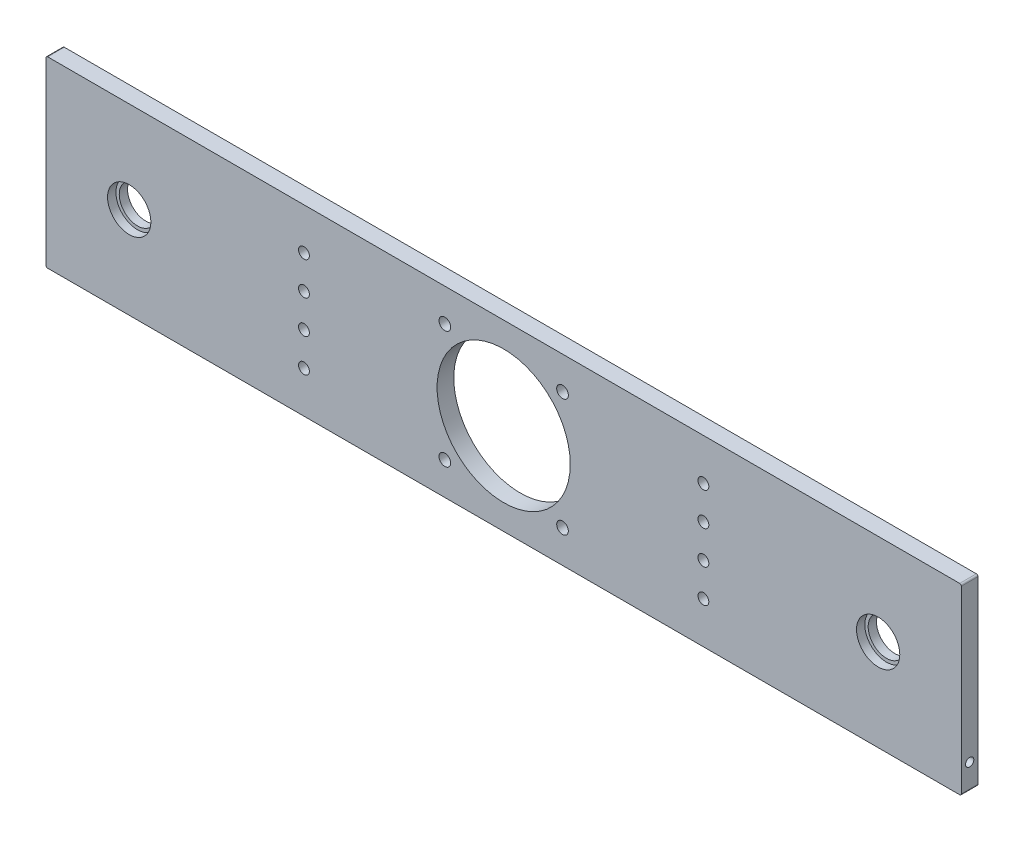
from build123d import *

# Parameters (mm, degrees)
SKETCH1_W           = 550
SKETCH1_H           = 110
BOSS_EXTRUDE1_DEPTH = 10
SKETCH3_R           = 13
CUT_EXTRUDE2_DEPTH  = 5
SKETCH4_R           = 11
CUT_EXTRUDE3_DEPTH  = 281.490641555
SKETCH5_R           = 40
CUT_EXTRUDE4_DEPTH  = 281.624304008
SKETCH6_R           = 3.5
CUT_EXTRUDE5_DEPTH  = 281.624304008
SKETCH7_R           = 3.25
CUT_EXTRUDE6_DEPTH  = 281.624304008
FILLET1_R           = 1


with BuildPart() as part:
    # Sketch1 → Boss-Extrude1 (new body)
    with BuildSketch(Plane.XY):
        Rectangle(SKETCH1_W, SKETCH1_H)
    extrude(amount=BOSS_EXTRUDE1_DEPTH)

    # Sketch3 → Cut-Extrude2 (cut)
    with BuildSketch(Plane.XY.offset(10)):
        with Locations((225, 0)):
            Circle(SKETCH3_R)
        with Locations(Location((-225, 0, 0), (0, 0, 180))):
            Circle(SKETCH3_R)
    extrude(amount=-CUT_EXTRUDE2_DEPTH, mode=Mode.SUBTRACT)

    # Sketch4 → Cut-Extrude3 (cut, through all)
    with BuildSketch(Plane.XY.offset(5)):
        with Locations((225, 0)):
            Circle(SKETCH4_R)
        with Locations(Location((-225, 0, 0), (0, 0, 180))):
            Circle(SKETCH4_R)
    extrude(amount=-CUT_EXTRUDE3_DEPTH, mode=Mode.SUBTRACT)

    # Sketch5 → Cut-Extrude4 (cut, through all)
    with BuildSketch(Plane.XY.offset(10)):
        Circle(SKETCH5_R)
    extrude(amount=-CUT_EXTRUDE4_DEPTH, mode=Mode.SUBTRACT)

    # Sketch6 → Cut-Extrude5 (cut, through all)
    with BuildSketch(Plane.XY.offset(10)):
        with Locations((-35.355339059, 35.355339059)):
            Circle(SKETCH6_R)
        with Locations((35.355339059, 35.355339059)):
            Circle(SKETCH6_R)
        with Locations((35.355339059, -35.355339059)):
            Circle(SKETCH6_R)
        with Locations((-35.355339059, -35.355339059)):
            Circle(SKETCH6_R)
    extrude(amount=-CUT_EXTRUDE5_DEPTH, mode=Mode.SUBTRACT)

    # Sketch7 → Cut-Extrude6 (cut, through all)
    with BuildSketch(Plane.XY.offset(10)):
        with Locations((-120, -10)):
            Circle(SKETCH7_R)
        with Locations((120, -10)):
            Circle(SKETCH7_R)
        with Locations((120, 10)):
            Circle(SKETCH7_R)
        with Locations((-120, 10)):
            Circle(SKETCH7_R)
        with Locations((-120, -30)):
            Circle(SKETCH7_R)
        with Locations((-120, 30)):
            Circle(SKETCH7_R)
        with Locations((120, 30)):
            Circle(SKETCH7_R)
        with Locations((120, -30)):
            Circle(SKETCH7_R)
    extrude(amount=-CUT_EXTRUDE6_DEPTH, mode=Mode.SUBTRACT)

    # Fillet1
    fillet1_edges = [part.edges().sort_by_distance(p)[0] for p in [
        (-275, 55, 5),
        (275, 55, 5),
        (275, -55, 5),
        (-275, -55, 5),
    ]]
    fillet(fillet1_edges, radius=FILLET1_R)

    # Sketch9 → M6 Tapped Hole1 (revolve, cut)
    with BuildSketch(Plane(origin=(-275, -40, 5), x_dir=(0, 0, 1), z_dir=(0, 1, 0))):
        Polygon((0, 0), (0, 19.502151548), (2.5, 18), (2.5, 0), align=None)
    m6_tapped_hole1 = revolve(axis=Axis((-281.35, -40, 5), (1, 0, 0)), mode=Mode.SUBTRACT)

    # Mirror1: M6 Tapped Hole1 across plane
    add(m6_tapped_hole1.mirror(Plane(origin=(0, 0, 0), x_dir=(0, 0, 1), z_dir=(1, 0, 0))), mode=Mode.SUBTRACT)


solid = part.part
